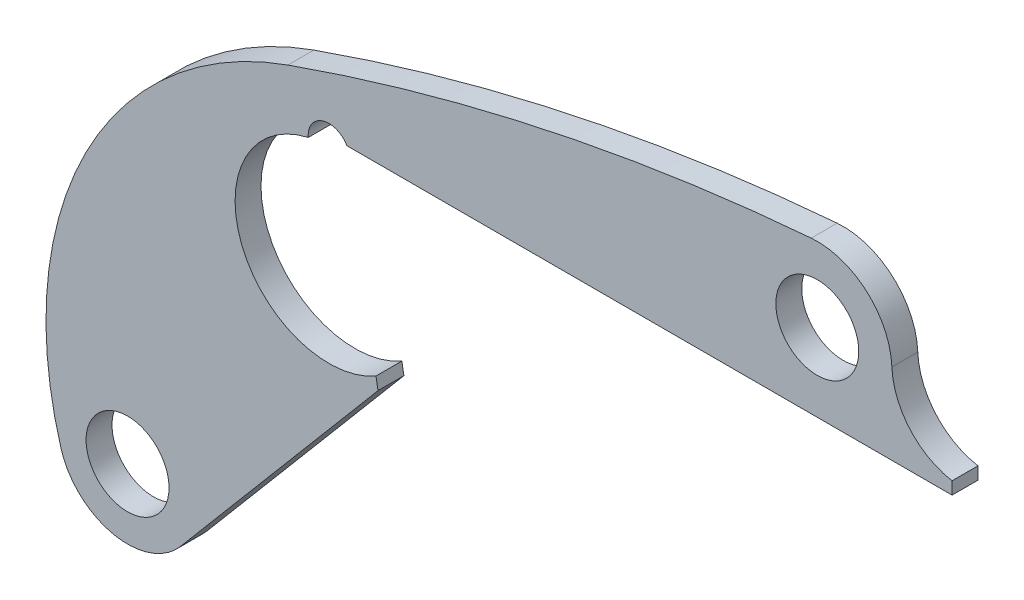
from build123d import *

# Parameters (mm, degrees)
SKETCH1_R           = 40
BOSS_EXTRUDE1_DEPTH = 25


with BuildPart() as part:
    # Sketch1 → Boss-Extrude1 (new body)
    with BuildSketch(Plane.XY):
        with BuildLine():
            Line((17.320508076, 100), (601, 100))
            Line((601, 100), (601, 112))
            ThreePointArc((601, 112), (560.305386081, 134.762632261), (542.936006728, 178.034952402))
            ThreePointArc((542.936006728, 178.034952402), (518.682115493, 228.948270242), (465.174941276, 246.763979062))
            ThreePointArc((465.174941276, 246.763979062), (209.331516914, 209.226035995), (-39.530360121, 138.99270262))
            ThreePointArc((-39.530360121, 138.99270262), (-234.732763539, -32.083318616), (-258.432243095, -290.558303887))
            ThreePointArc((-258.432243095, -290.558303887), (-207.948857392, -337.074148263), (-143.032705856, -314.75399415))
            Line((-143.032705856, -314.75399415), (47.3, -89.6))
            Line((47.3, -89.6), (45.380171882, -78.3))
            ThreePointArc((45.380171882, -78.3), (-84.25636808, -33.032021404), (-19.925830789, 88.279166667))
            ThreePointArc((-19.925830789, 88.279166667), (-6.003449851, 109.077698758), (17.320508076, 100))
        make_face()
        with Locations((-194.2, -271.5)):
            Circle(SKETCH1_R, mode=Mode.SUBTRACT)
        with Locations((471, 175)):
            Circle(SKETCH1_R, mode=Mode.SUBTRACT)
    extrude(amount=BOSS_EXTRUDE1_DEPTH)


solid = part.part
